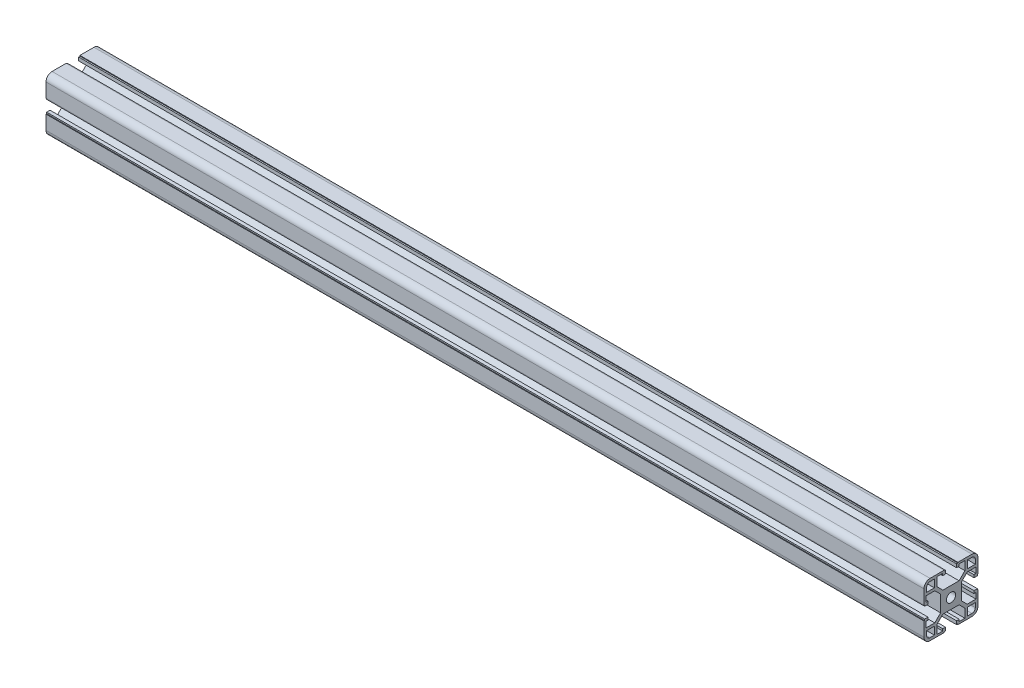
from build123d import *

# Parameters (mm, degrees)
SKETCH1_R                                 = 3.4
ALUMINIUM_PROFILE_40_X_40B_X_R4_5_1_DEPTH = 650


with BuildPart() as part:
    # Sketch1 → Aluminium profile 40 X 40B X R4.5(1) (new body)
    with BuildSketch(Plane.YZ.offset(-984.974958264)):
        with BuildLine():
            Line((-5.1, 20), (-5.1, 19.5))
            Line((-5.1, 19.5), (-4.1, 19.5))
            Line((-4.1, 19.5), (-4.1, 17))
            Line((-4.1, 17), (-6.1, 17))
            Line((-6.1, 17), (-6.1, 18.5))
            Line((-6.1, 18.5), (-10.3, 18.5))
            Line((-10.3, 18.5), (-10.3, 12))
            Line((-10.3, 12), (-6, 7.7))
            Line((-6, 7.7), (6, 7.7))
            Line((6, 7.7), (10.3, 12))
            Line((10.3, 12), (10.3, 18.5))
            Line((10.3, 18.5), (6.1, 18.5))
            Line((6.1, 18.5), (6.1, 17))
            Line((6.1, 17), (4.1, 17))
            Line((4.1, 17), (4.1, 19.5))
            Line((4.1, 19.5), (5.1, 19.5))
            Line((5.1, 19.5), (5.1, 20))
            Line((5.1, 20), (15.5, 20))
            ThreePointArc((15.5, 20), (18.681980515, 18.681980515), (20, 15.5))
            Line((20, 15.5), (20, 5.1))
            Line((20, 5.1), (19.5, 5.1))
            Line((19.5, 5.1), (19.5, 4.1))
            Line((19.5, 4.1), (17, 4.1))
            Line((17, 4.1), (17, 6.1))
            Line((17, 6.1), (18.5, 6.1))
            Line((18.5, 6.1), (18.5, 10.3))
            Line((18.5, 10.3), (12, 10.3))
            Line((12, 10.3), (7.7, 6))
            Line((7.7, 6), (7.7, -6))
            Line((7.7, -6), (12, -10.3))
            Line((12, -10.3), (18.5, -10.3))
            Line((18.5, -10.3), (18.5, -6.1))
            Line((18.5, -6.1), (17, -6.1))
            Line((17, -6.1), (17, -4.1))
            Line((17, -4.1), (19.5, -4.1))
            Line((19.5, -4.1), (19.5, -5.1))
            Line((19.5, -5.1), (20, -5.1))
            Line((20, -5.1), (20, -15.5))
            ThreePointArc((20, -15.5), (18.681980515, -18.681980515), (15.5, -20))
            Line((15.5, -20), (5.1, -20))
            Line((5.1, -20), (5.1, -19.5))
            Line((5.1, -19.5), (4.1, -19.5))
            Line((4.1, -19.5), (4.1, -17))
            Line((4.1, -17), (6.1, -17))
            Line((6.1, -17), (6.1, -18.5))
            Line((6.1, -18.5), (10.3, -18.5))
            Line((10.3, -18.5), (10.3, -12))
            Line((10.3, -12), (6, -7.7))
            Line((6, -7.7), (-6, -7.7))
            Line((-6, -7.7), (-10.3, -12))
            Line((-10.3, -12), (-10.3, -18.5))
            Line((-10.3, -18.5), (-6.1, -18.5))
            Line((-6.1, -18.5), (-6.1, -17))
            Line((-6.1, -17), (-4.1, -17))
            Line((-4.1, -17), (-4.1, -19.5))
            Line((-4.1, -19.5), (-5.1, -19.5))
            Line((-5.1, -19.5), (-5.1, -20))
            Line((-5.1, -20), (-15.5, -20))
            ThreePointArc((-15.5, -20), (-18.681980515, -18.681980515), (-20, -15.5))
            Line((-20, -15.5), (-20, -5.1))
            Line((-20, -5.1), (-19.5, -5.1))
            Line((-19.5, -5.1), (-19.5, -4.1))
            Line((-19.5, -4.1), (-17, -4.1))
            Line((-17, -4.1), (-17, -6.1))
            Line((-17, -6.1), (-18.5, -6.1))
            Line((-18.5, -6.1), (-18.5, -10.3))
            Line((-18.5, -10.3), (-12, -10.3))
            Line((-12, -10.3), (-7.7, -6))
            Line((-7.7, -6), (-7.7, 6))
            Line((-7.7, 6), (-12, 10.3))
            Line((-12, 10.3), (-18.5, 10.3))
            Line((-18.5, 10.3), (-18.5, 6.1))
            Line((-18.5, 6.1), (-17, 6.1))
            Line((-17, 6.1), (-17, 4.1))
            Line((-17, 4.1), (-19.5, 4.1))
            Line((-19.5, 4.1), (-19.5, 5.1))
            Line((-19.5, 5.1), (-20, 5.1))
            Line((-20, 5.1), (-20, 15.5))
            ThreePointArc((-20, 15.5), (-18.681980515, 18.681980515), (-15.5, 20))
            Line((-15.5, 20), (-5.1, 20))
        make_face()
        Circle(SKETCH1_R, mode=Mode.SUBTRACT)
        with BuildLine():
            Line((12.3, 18), (15.5, 18))
            ThreePointArc((15.5, 18), (17.267766953, 17.267766953), (18, 15.5))
            Line((18, 15.5), (18, 12.3))
            Line((18, 12.3), (12.3, 12.3))
            Line((12.3, 12.3), (12.3, 18))
        make_face(mode=Mode.SUBTRACT)
        with BuildLine():
            Line((-15.5, 18), (-12.3, 18))
            Line((-12.3, 18), (-12.3, 12.3))
            Line((-12.3, 12.3), (-18, 12.3))
            Line((-18, 12.3), (-18, 15.5))
            ThreePointArc((-18, 15.5), (-17.267766953, 17.267766953), (-15.5, 18))
        make_face(mode=Mode.SUBTRACT)
        with BuildLine():
            Line((-18, -12.3), (-12.3, -12.3))
            Line((-12.3, -12.3), (-12.3, -18))
            Line((-12.3, -18), (-15.5, -18))
            ThreePointArc((-15.5, -18), (-17.267766953, -17.267766953), (-18, -15.5))
            Line((-18, -15.5), (-18, -12.3))
        make_face(mode=Mode.SUBTRACT)
        with BuildLine():
            Line((12.3, -12.3), (18, -12.3))
            Line((18, -12.3), (18, -15.5))
            ThreePointArc((18, -15.5), (17.267766953, -17.267766953), (15.5, -18))
            Line((15.5, -18), (12.3, -18))
            Line((12.3, -18), (12.3, -12.3))
        make_face(mode=Mode.SUBTRACT)
    extrude(amount=ALUMINIUM_PROFILE_40_X_40B_X_R4_5_1_DEPTH)


solid = part.part
